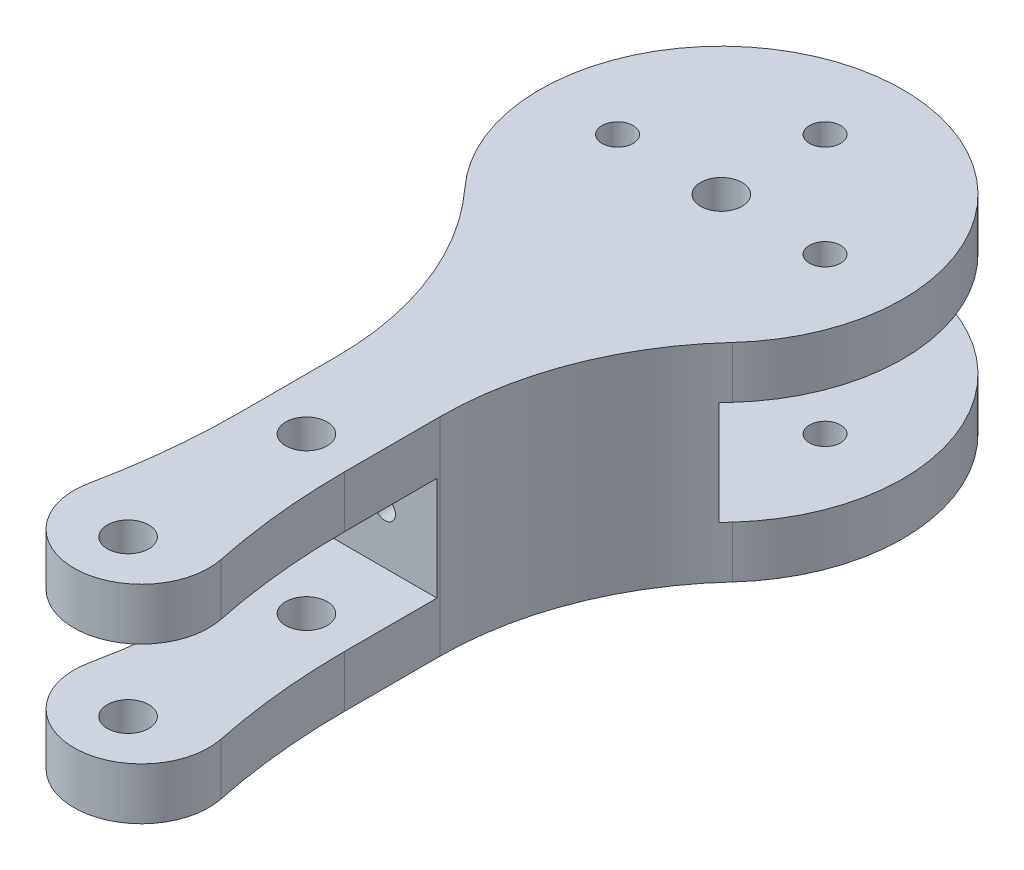
from build123d import *

# Parameters (mm, degrees)
BOSS_EXTRUDE1_DEPTH     = 20
CUT_EXTRUDE1_DEPTH      = 68.837474407
CUT_EXTRUDE1_DEPTH_BACK = 68.837474407
SKETCH2_R               = 2
SKETCH3_R               = 2
CUT_EXTRUDE2_DEPTH      = 68.837474407
SKETCH4_R               = 1.5
CUT_EXTRUDE3_DEPTH      = 68.837474407
CUT_EXTRUDE4_DEPTH      = 68.837474407
CUT_EXTRUDE4_DEPTH_BACK = 68.837474407
SKETCH5_W               = 30
SKETCH5_H               = 10
SKETCH6_R               = 6
BOSS_EXTRUDE2_DEPTH     = 5
SKETCH7_R               = 2
BOSS_EXTRUDE4_DEPTH     = 10
SKETCH8_R               = 1
CUT_EXTRUDE5_DEPTH      = 30


with BuildPart() as part:
    # Sketch1 → Boss-Extrude1 (new body)
    with BuildSketch(Plane(origin=(0, 0, 0), x_dir=(1, 0, 0), z_dir=(0, 1, 0))):
        with BuildLine():
            Line((-5, -32.113081447), (-5, -41.34652383))
            ThreePointArc((-5, -41.34652383), (-5.341807803, -48.003714064), (-6.363636364, -54.590889543))
            ThreePointArc((-6.363636364, -54.590889543), (0, -62.415326114), (6.363636364, -54.590889543))
            ThreePointArc((6.363636364, -54.590889543), (5.341807803, -48.003714064), (5, -41.34652383))
            Line((5, -41.34652383), (5, -32.113081447))
            ThreePointArc((5, -32.113081447), (7.043266511, -21.230937695), (12.894736842, -11.83113527))
            ThreePointArc((12.894736842, -11.83113527), (0, 17.5), (-12.894736842, -11.83113527))
            ThreePointArc((-12.894736842, -11.83113527), (-7.043266511, -21.230937695), (-5, -32.113081447))
        make_face()
    extrude(amount=BOSS_EXTRUDE1_DEPTH)

    # Sketch2 → Cut-Extrude1 (cut, two sides: drawn at the far end of the back side and taken through both)
    with BuildSketch(Plane(origin=(0, 20, 0), x_dir=(1, 0, 0), z_dir=(0, 1, 0)).offset(-CUT_EXTRUDE1_DEPTH_BACK)):
        with Locations(Location((0, -40, 0), (0, 0, 270))):
            Circle(SKETCH2_R)
        with Locations(Location((0, -57.194020253, 0), (0, 0, 270))):
            Circle(SKETCH2_R)
    extrude(amount=CUT_EXTRUDE1_DEPTH + CUT_EXTRUDE1_DEPTH_BACK, mode=Mode.SUBTRACT)

    # Sketch3 → Cut-Extrude2 (cut, through all)
    with BuildSketch(Plane(origin=(0, 20, 0), x_dir=(1, 0, 0), z_dir=(0, 1, 0))):
        with Locations(Location((0, 0, 0), (0, 0, 270))):
            Circle(SKETCH3_R)
    extrude(amount=-CUT_EXTRUDE2_DEPTH, mode=Mode.SUBTRACT)

    # Sketch4 → Cut-Extrude3 (cut, through all)
    with BuildSketch(Plane(origin=(0, 20, 0), x_dir=(1, 0, 0), z_dir=(0, 1, 0))):
        with Locations(Location((-10, 0, 0), (0, 0, 270))):
            Circle(SKETCH4_R)
        with Locations(Location((10, 0, 0), (0, 0, 270))):
            Circle(SKETCH4_R)
        with Locations(Location((0, 10, 0), (0, 0, 270))):
            Circle(SKETCH4_R)
    extrude(amount=-CUT_EXTRUDE3_DEPTH, mode=Mode.SUBTRACT)

    # Sketch5 → Cut-Extrude4 (cut, two sides: drawn at the far end of the back side and taken through both)
    with BuildSketch(Plane(origin=(0, 0, 0), x_dir=(0, 0, -1), z_dir=(1, 0, 0)).offset(-CUT_EXTRUDE4_DEPTH_BACK)):
        with Locations((-47.415326114, 10)):
            Rectangle(SKETCH5_W, SKETCH5_H)
        with Locations((2.5, 10)):
            Rectangle(SKETCH5_W, SKETCH5_H)
    extrude(amount=CUT_EXTRUDE4_DEPTH + CUT_EXTRUDE4_DEPTH_BACK, mode=Mode.SUBTRACT)

    # Sketch6 → Boss-Extrude2 (add)
    with BuildSketch(Plane.XZ):
        with Locations(Location((0, 0, 0), (0, 0, 270))):
            Circle(SKETCH6_R)
    extrude(amount=BOSS_EXTRUDE2_DEPTH)

    # Sketch8 → Cut-Extrude5 (cut)
    with BuildSketch(Plane(origin=(0, 0, 12.5), x_dir=(-1, 0, 0), z_dir=(0, 0, -1))):
        with Locations((0, 9.975810979)):
            Circle(SKETCH8_R)
    extrude(amount=-CUT_EXTRUDE5_DEPTH, mode=Mode.SUBTRACT)


with BuildPart() as body_2:
    # Sketch7 → Boss-Extrude4 (new body)
    with BuildSketch(Plane(origin=(0, 5, 0), x_dir=(1, 0, 0), z_dir=(0, 1, 0))):
        with Locations(Location((0, 0, 0), (0, 0, 270))):
            Circle(SKETCH7_R)
    extrude(amount=BOSS_EXTRUDE4_DEPTH)


solid = Compound([part.part, body_2.part])
